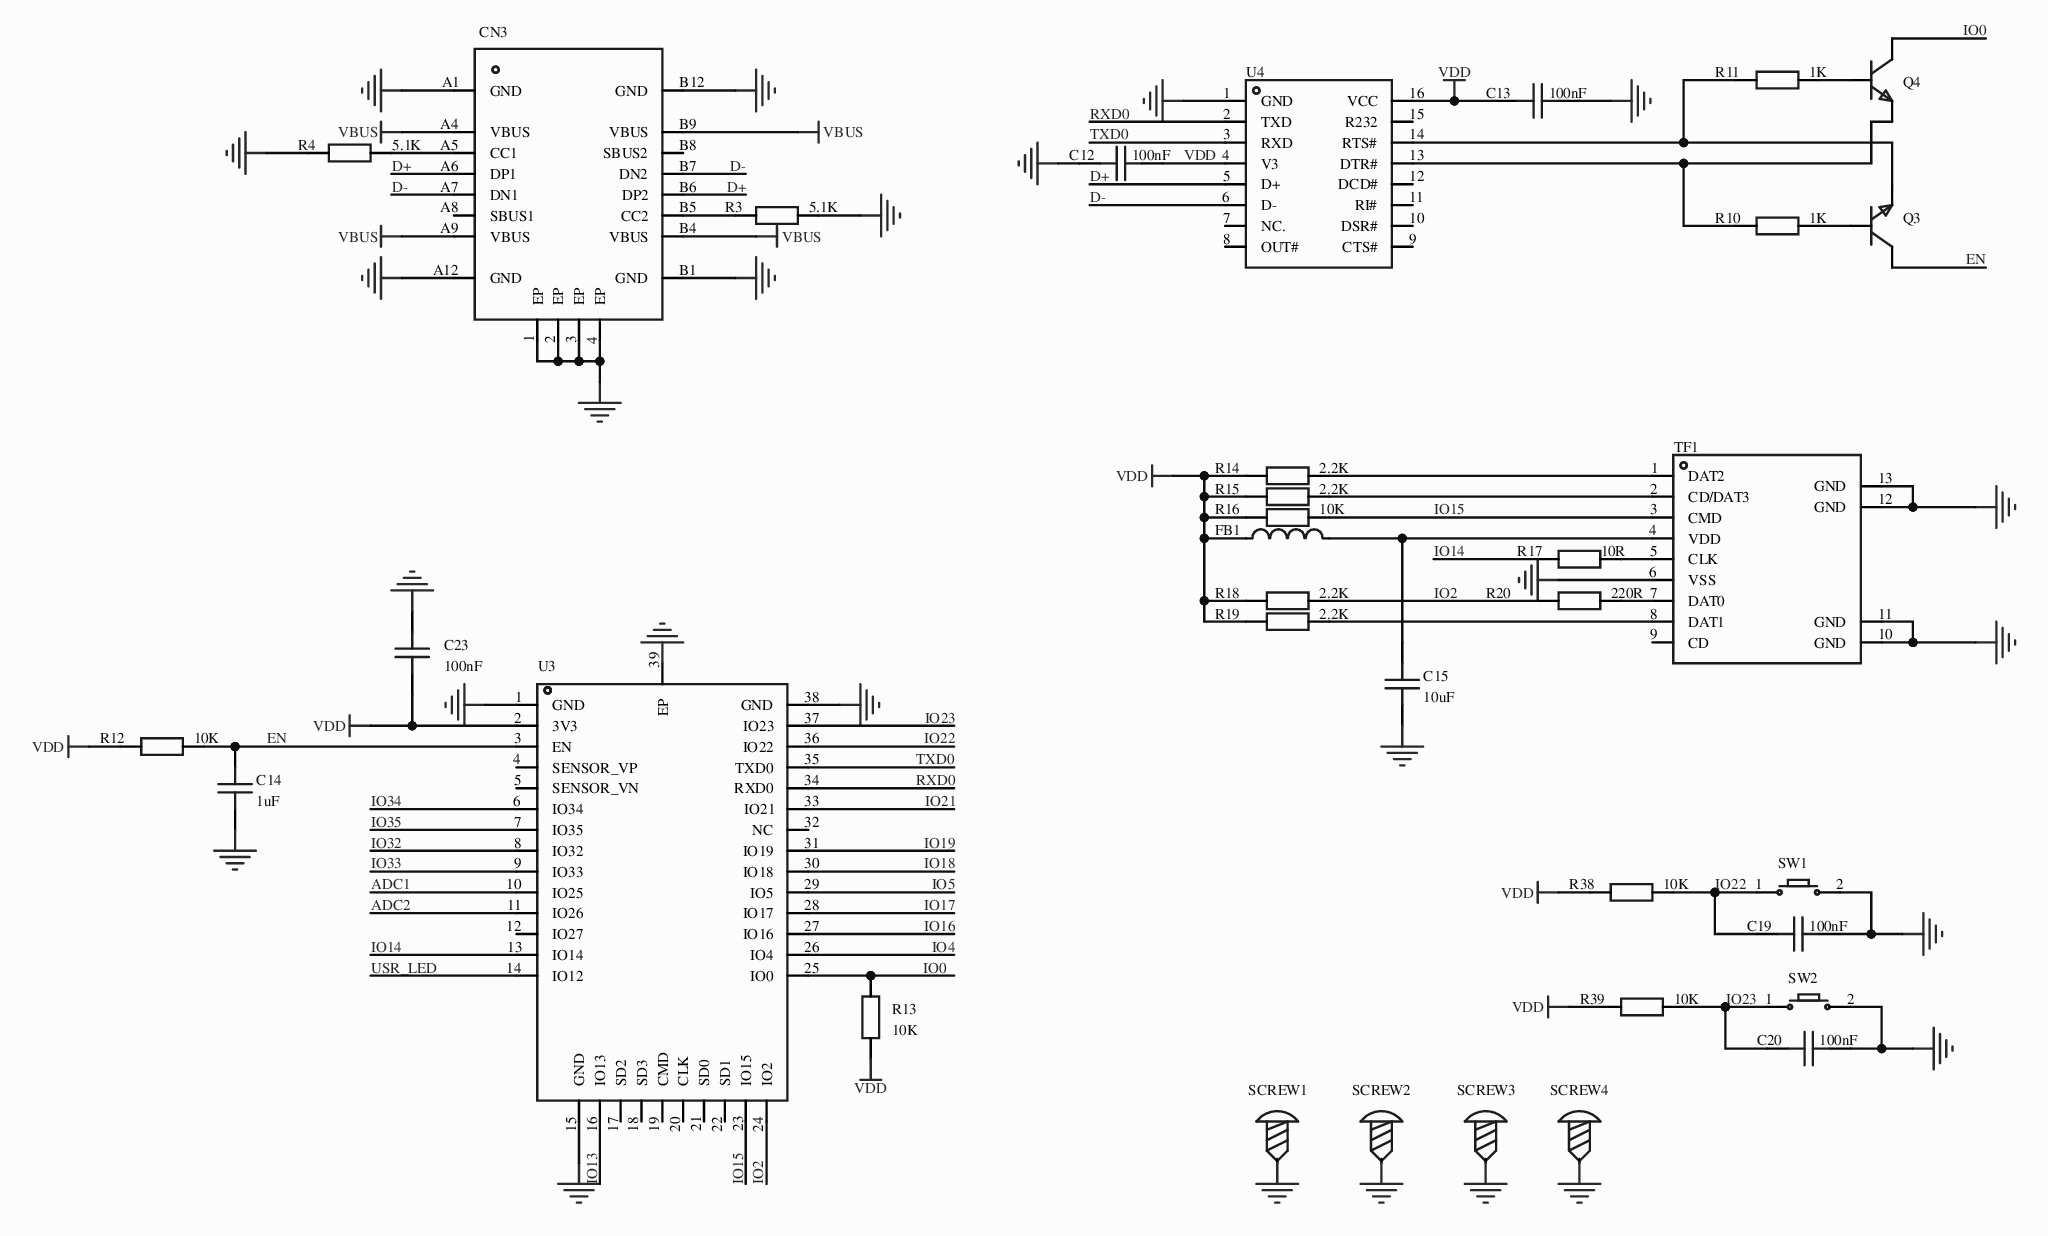
[diagram p0: MISC49869-4.schdoc]
# Altium project MISC49869-2.PrjPcb
3 sheets, 114 parts. Net scope: global (net labels, ports and power ports of the same name join across sheets).
Board file: MISC49869.pcbdoc
Sheets:
  MISC49869-4.schdoc
  MISC49869-3.schdoc
  MISC49869-5.schdoc

## Sheet MISC49869-4.schdoc
size 297 x 209 mm; @Create Time: 11:47:24; @Update Time: 11:51:06; @Board Name: MISC49869; Version: V1.0; @Project Name: MISC49869; @Page Count: 3; @Update Date: 2026-04-07; @Create Date: 2026-04-07; @Schematic Name: MISC49869; @Page No: 1

### Parts
C12  value 100nF  [C0805]  (hidden comment: CAP_0805)
C13  value 100nF  [C0805]  (hidden comment: CAP_0805)
C14  value 1uF  [C0805]  (hidden comment: CAP_0805)
C15  value 10uF  [C0805]  (hidden comment: CAP_0805)
C19  value 100nF  [C0805]  (hidden comment: CAP_0805)
C20  value 100nF  [C0805]  (hidden comment: CAP_0805)
C23  value 100nF  [C0805]  (hidden comment: CAP_0805)
CN3  USB_TYPE-C-16P  [USB_TYPE-C-16P]  (value not drawn)
FB1  L_0805  [L0805]  (value not drawn)
Q3  SS8050_C7420370  [SOT-23-3_L2.9-W1.3-P1.90-LS2.4-BR]  (value not drawn)
Q4  SS8050_C7420370  [SOT-23-3_L2.9-W1.3-P1.90-LS2.4-BR]  (value not drawn)
R3  value 5.1K  [R0805]  (hidden comment: Res_0805)
R4  value 5.1K  [R0805]  (hidden comment: Res_0805)
R10  value 1K  [R0805]  (hidden comment: Res_0805)
R11  value 1K  [R0805]  (hidden comment: Res_0805)
R12  value 10K  [R0805]  (hidden comment: Res_0805)
R13  value 10K  [R0805]  (hidden comment: Res_0805)
R14  value 2.2K  [R0805]  (hidden comment: Res_0805)
R15  value 2.2K  [R0805]  (hidden comment: Res_0805)
R16  value 10K  [R0805]  (hidden comment: Res_0805)
R17  value 10R  [R0805]  (hidden comment: Res_0805)
R18  value 2.2K  [R0805]  (hidden comment: Res_0805)
R19  value 2.2K  [R0805]  (hidden comment: Res_0805)
R20  value 220R  [R0805]  (hidden comment: Res_0805)
R38  value 10K  [R0805]  (hidden comment: Res_0805)
R39  value 10K  [R0805]  (hidden comment: Res_0805)
SCREW1  M2 screw  [M2螺丝]  (value not drawn)
SCREW2  M2 screw  [M2螺丝]  (value not drawn)
SCREW3  M2 screw  [M2螺丝]  (value not drawn)
SCREW4  M2 screw  [M2螺丝]  (value not drawn)
SW1  Key_SMD_3x4x2  [Key_SMD_3x4x2]  (value not drawn)
SW2  Key_SMD_3x4x2  [Key_SMD_3x4x2]  (value not drawn)
TF1  TF-CARD H1.8  [TF-SMD_TF-CARD-H1.8]  (value not drawn)
U3  ESP32-WROOM-32  [WIFIM-SMD_ESP-WROOM-32]  (value not drawn)
U4  CH340C  [SOP-16_L10.0-W3.9-P1.27-LS6.0-BL]  (value not drawn)

### Nets
GND: C12.2 C13.1 C14.2 C15.2 C19.1 C20.1 C23.2 CN3.1(EP) CN3.2(EP) CN3.3(EP) CN3.4(EP) CN3.A1(GND) CN3.A12(GND) CN3.B1(GND) CN3.B12(GND) R3.1 R4.1 SCREW1.1 SCREW2.1 SCREW3.1 SCREW4.1 SW1.2 SW2.2 TF1.6(VSS) TF1.10(GND) TF1.11(GND) TF1.12(GND) TF1.13(GND) U3.1(GND) U3.15(GND) U3.38(GND) U3.39(EP) U4.1(GND)
VBUS: CN3.A4(VBUS) CN3.A9(VBUS) CN3.B4(VBUS) CN3.B9(VBUS)
VDD: C12.1 C13.2 C23.1 FB1.1 R12.2 R13.2 R14.2 R15.2 R16.2 R18.2 R19.2 R38.2 R39.2 U3.2(3V3) U4.4(V3) U4.16(VCC)
ADC1: U3.10(IO25)
ADC2: U3.11(IO26)
D+: CN3.A6(DP1) CN3.B6(DP2) U4.5(D+)
D-: CN3.A7(DN1) CN3.B7(DN2) U4.6(D-)
EN: C14.1 Q3.3(C) R12.1 U3.3(EN)
IO0: Q4.3(C) R13.1 U3.25(IO0)
IO2: R18.1 R20.2 U3.24(IO2)
IO4: U3.26(IO4)
IO5: U3.29(IO5)
IO13: U3.16(IO13)
IO14: R17.2 U3.13(IO14)
IO15: R16.1 TF1.3(CMD) U3.23(IO15)
IO16: U3.27(IO16)
IO17: U3.28(IO17)
IO18: U3.30(IO18)
IO19: U3.31(IO19)
IO21: U3.33(IO21)
IO22: C19.2 R38.1 SW1.1 U3.36(IO22)
IO23: C20.2 R39.1 SW2.1 U3.37(IO23)
IO32: U3.8(IO32)
IO33: U3.9(IO33)
IO34: U3.6(IO34)
IO35: U3.7(IO35)
RXD0: U3.34(RXD0) U4.2(TXD)
TXD0: U3.35(TXD0) U4.3(RXD)
USR_LED: U3.14(IO12)
NetC15_1: C15.1 FB1.2 TF1.4(VDD)
NetCN3_A5: CN3.A5(CC1) R4.2
NetCN3_B5: CN3.B5(CC2) R3.2
NetQ3_1: Q3.1(B) R10.1
NetQ3_2: Q3.2(E) R11.2 U4.14(RTS#)
NetQ4_1: Q4.1(B) R11.1
NetQ4_2: Q4.2(E) R10.2 U4.13(DTR#)
NetR14_1: R14.1 TF1.1(DAT2)
NetR15_1: R15.1 TF1.2(CD/DAT3)
NetR17_1: R17.1 TF1.5(CLK)
NetR19_1: R19.1 TF1.8(DAT1)
NetR20_1: R20.1 TF1.7(DAT0)

Not connected (* = marked no-connect by the designer): CN3 A8(SBUS1)* B8(SBUS2)*; TF1 9(CD)*; U3 4(SENSOR_VP)* 5(SENSOR_VN)* 12(IO27)* 17(SD2)* 18(SD3)* 19(CMD)* 20(CLK)* 21(SD0)* 22(SD1)* 32(NC)*; U4 7(NC.)* 8(OUT#)* 9(CTS#)* 10(DSR#)* 11(RI#)* 12(DCD#)* 15(R232)*

### Library data of the parts
C12-C15 C19 C20 C23 = CAP_0805: ConvertToPcb: yes; SymbolName: CapAcitance; ModelId: 1ba041120af144c991958decab20d241; ModelName: C0805_L2.0-W1.3-H1.3; ModelTransform: 78.74,51.181,0,0,0,0,0,0.0005,0; Device: CAP_0805; AddInBom: yes; FootprintName: C0805
CN3 = USB_TYPE-C-16P: AddInBom: yes; ModelId: 35058e297fd54ee2afd2de30c3ce7155; ModelName: USB-C_SMD-TYPE-C-31-M-12; ModelTransform: 360,318.121,0,180,0,0,0,-41.02,-39.37; Device: USB_TYPE-C-16P; ConvertToPcb: yes; SymbolName: USB_TYPE-C-16P; FootprintName: USB_TYPE-C-16P
FB1 = L_0805: Symbol: SDFL2012S100KTF; Value: 10uH; AddInBom: yes; ModelId: 37a81e68749a4138bd2dfa6897b24b85; ModelName: R0805_L2.0-W1.3-H0.6; ModelTransform: 78.74,51.181,0,0,0,0,0,0.001,0; Device: L_0805; ConvertToPcb: yes; FootprintName: L0805
Q3 Q4 = SS8050_C7420370: AddInBom: yes; ModelId: c62791f0466c4ae2a892c056b845b0ca; ModelName: SOT-23-3P_L2.9-W1.3-H1.0-LS2.4-P0.95; ModelTransform: 98.425,114.173,0,180,0,0,0.0005,-0.0005,0; Symbol: SS8050_C7420370; Device: SS8050_C7420370; ConvertToPcb: yes; FootprintName: SOT-23-3_L2.9-W1.3-P1.90-LS2.4-BR
R3 R4 R10-R20 R38 R39 = Res_0805: ConvertToPcb: yes; SymbolName: Resistor; ModelId: 37a81e68749a4138bd2dfa6897b24b85; ModelName: R0805_L2.0-W1.3-H0.6; ModelTransform: 78.74,51.181,0,0,0,0,0,-0.0005,0; Device: Res_0805; AddInBom: yes; FootprintName: R0805
SCREW1-SCREW4 = M2螺丝: ConvertToPcb: yes; SymbolName: Screw hole; Device: M2 screw; AddInBom: yes; FootprintName: M2 screw
SW1 SW2 = Key_SMD_3x4x2: ConvertToPcb: yes; SymbolName: Tact switch x2; ModelId: 63599cce708d48afbce1b0db003544770819f05c4eef4c71ace90d822a990e87; ModelName: SW-SMD_L4.0-W2.9-H2-LS5.0; ModelTransform: 196.85,114.17,79.13,0,0,0,0,0,0; Device: Key_SMD_3x4x2; AddInBom: yes; FootprintName: Key_SMD_3x4x2
TF1 = TF-CARD H1.8: AddInBom: yes; ModelId: 9b9c093eaf784fafb0b50515d8d92d39; ModelTransform: 631.8885,594.487,0,0,0,0,-0.002,-75.432,-23.622; Symbol: TF-CARD H1.8; Device: TF-CARD H1.8; ConvertToPcb: yes; FootprintName: TF-SMD_TF-CARD-H1.8; ModelName: TF-SMD_TF-CARD-H1.8
U3 = ESP32-WROOM-32: Symbol: ESP-WROOM-32; AddInBom: yes; ModelId: 5a2678a0bdc04ba384e1e7621568aeee; ModelName: WIFIM-SMD_L25.5-W18.0-H3.1; ModelTransform: 709.4474,1004.3287,0,0,0,0,0,145.633,0; Device: ESP32-WROOM-32; ConvertToPcb: yes; FootprintName: WIFIM-SMD_ESP-WROOM-32
U4 = CH340C: AddInBom: yes; ModelId: 3361a6792abf4a8f8fbca4f1924a67ee; ModelName: SOP-16_L9.9-W3.9-H1.5-LS6.0-P1.27; ModelTransform: 240.39054,393.7,0,90,0,0,0,0,0; Symbol: CH340C; Device: CH340C; ConvertToPcb: yes; FootprintName: SOP-16_L10.0-W3.9-P1.27-LS6.0-BL

## Sheet MISC49869-3.schdoc
size 297 x 209 mm; @Create Time: 11:47:24; @Update Time: 09:47:04; @Board Name: MISC49869; Version: V1.0; @Project Name: MISC49869; @Page Count: 3; @Update Date: 2026-04-07; @Create Date: 2026-04-07; @Schematic Name: MISC49869; @Page No: 2
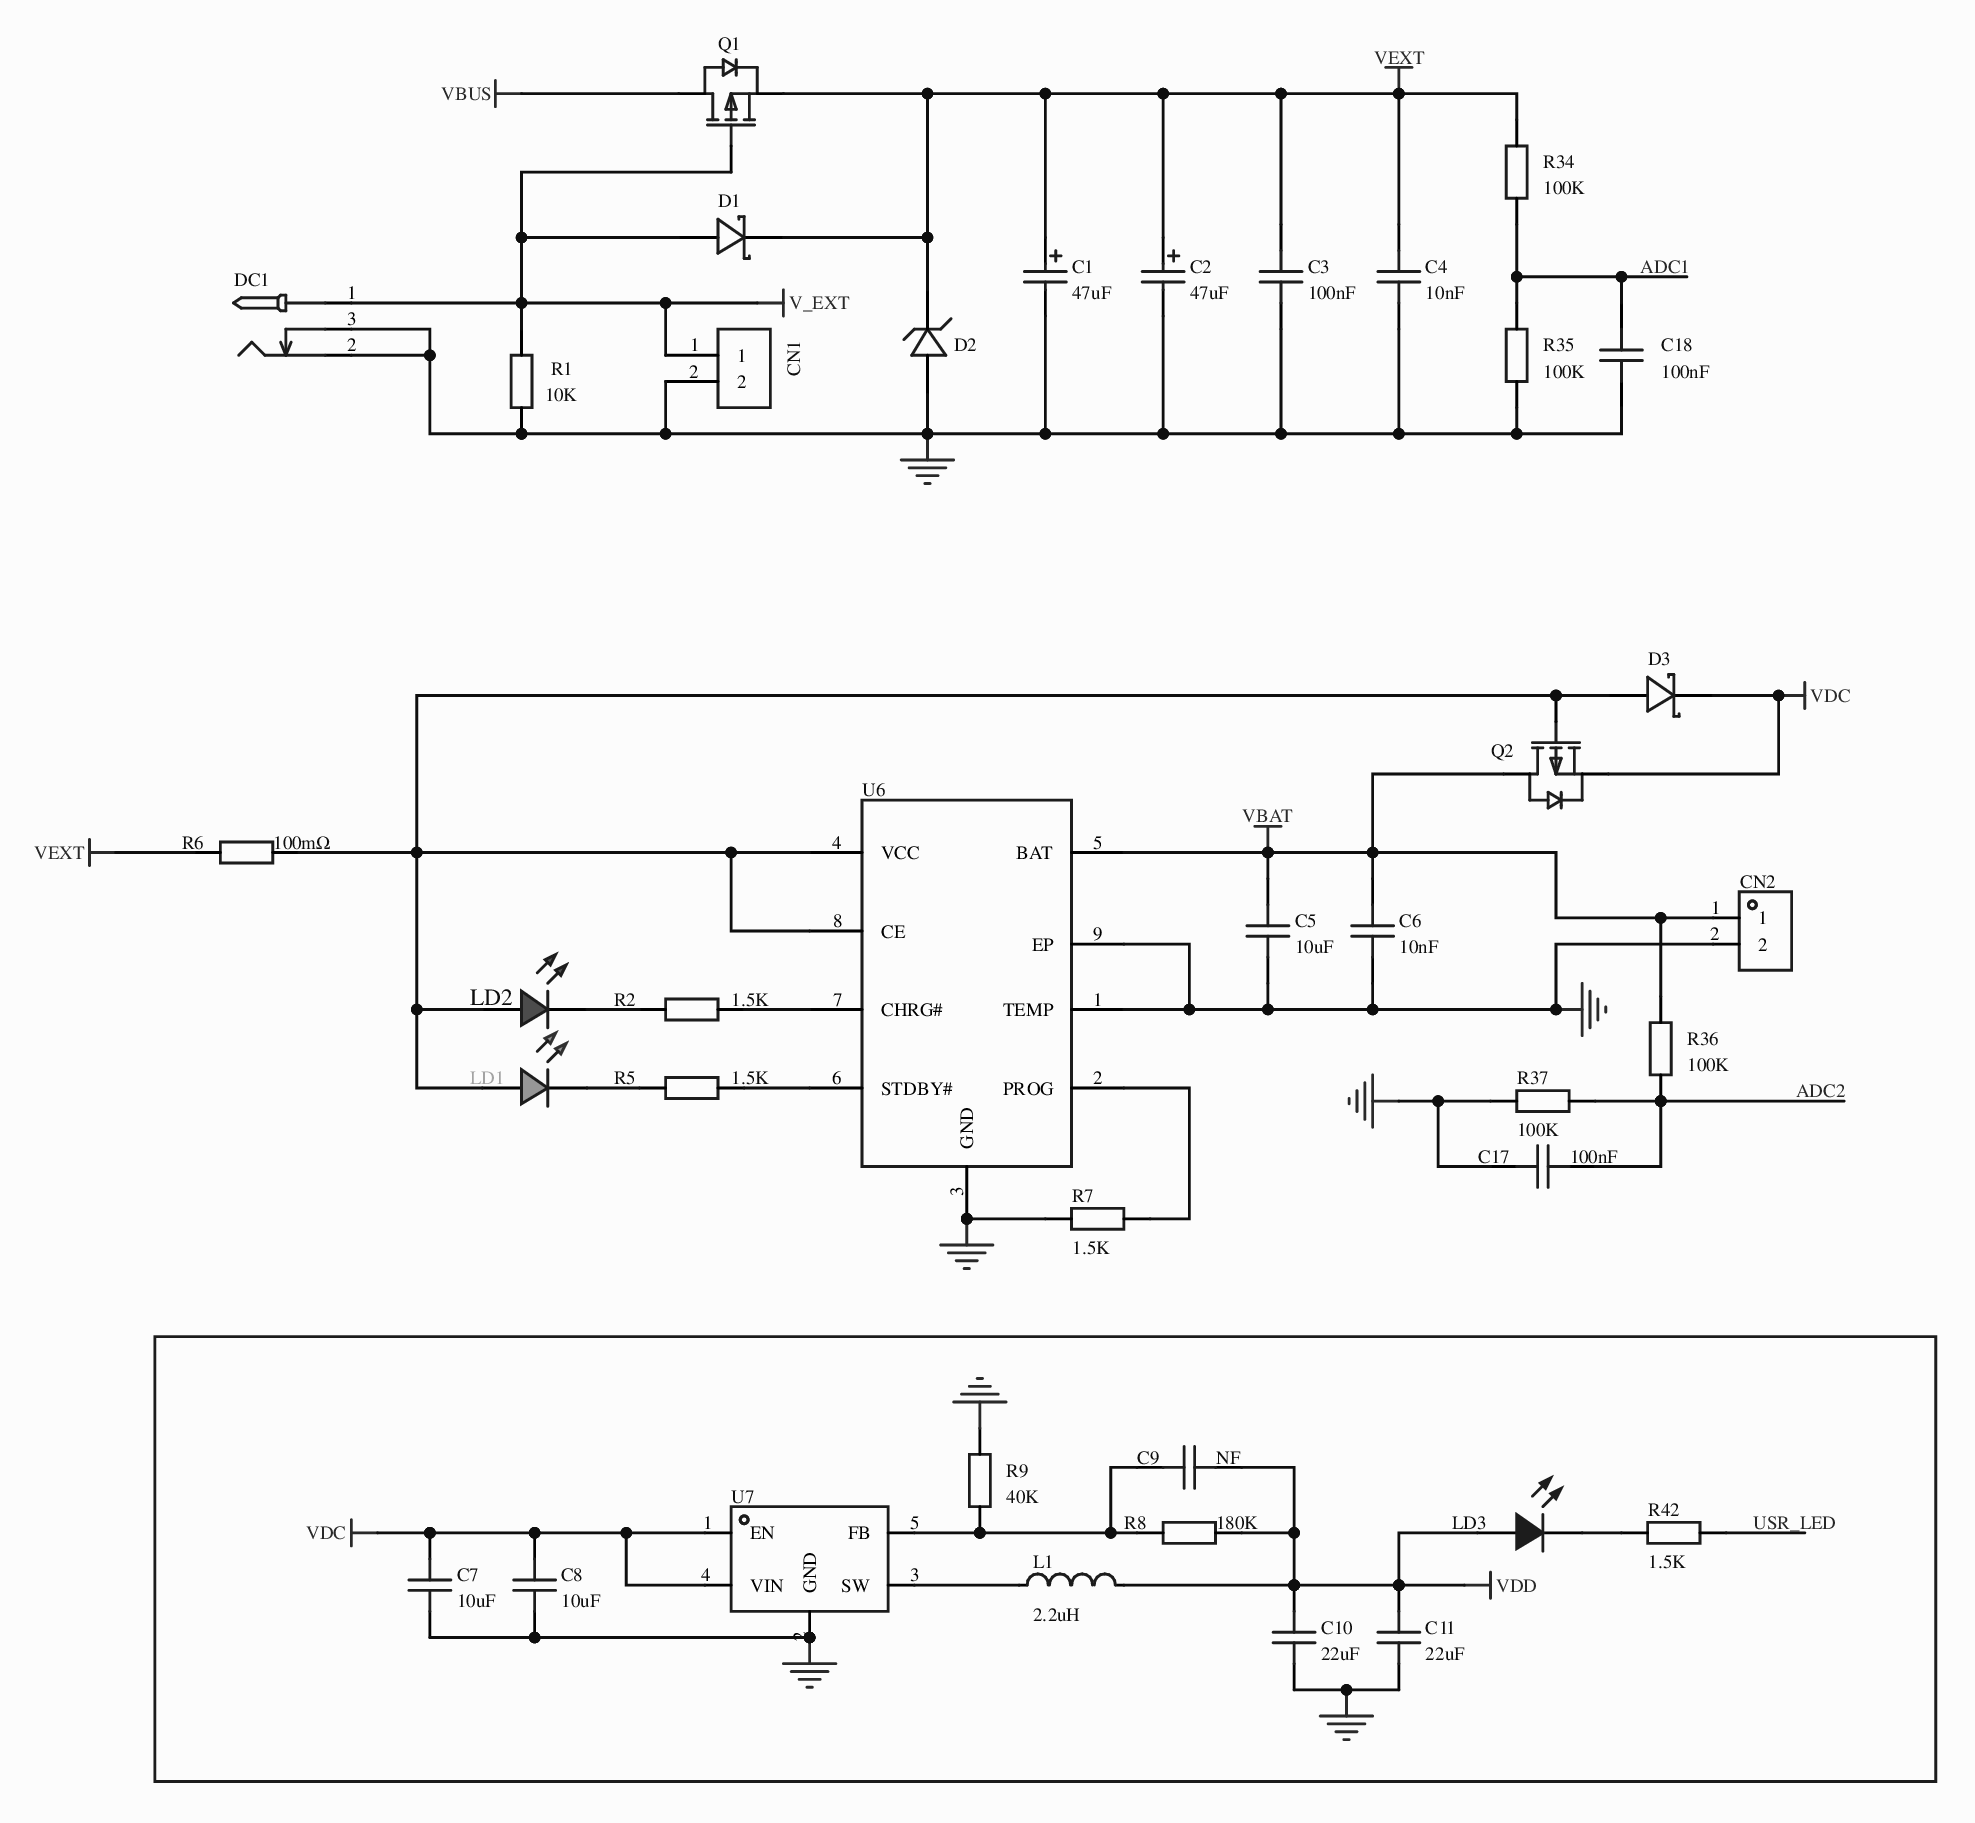
[diagram p1: MISC49869-3.schdoc]

### Parts
C1  value 47uF  [C_Ele_SMD_4x5.5mm]  (hidden comment: C_Ele_SMD_5x5.4mm)
C2  value 47uF  [C_Ele_SMD_4x5.5mm]  (hidden comment: C_Ele_SMD_5x5.4mm)
C3  value 100nF  [C0805]  (hidden comment: CAP_0805)
C4  value 10nF  [C0805]  (hidden comment: CAP_0805)
C5  value 10uF  [C0805]  (hidden comment: CAP_0805)
C6  value 10nF  [C0805]  (hidden comment: CAP_0805)
C7  value 10uF  [C0805]  (hidden comment: CAP_0805)
C8  value 10uF  [C0805]  (hidden comment: CAP_0805)
C9  value NF  [C0805]  (hidden comment: CAP_0805)
C10  value 22uF  [C0805]  (hidden comment: CAP_0805)
C11  value 22uF  [C0805]  (hidden comment: CAP_0805)
C17  value 100nF  [C0805]  (hidden comment: CAP_0805)
C18  value 100nF  [C0805]  (hidden comment: CAP_0805)
CN1  WJ500V-5.08-2P  [CONN-TH_2P-P5.00_WJ500V-5.08-2P]  (value not drawn)
CN2  ZX-XH2.54-2PZZ  [CONN-TH_2P-P2.50_HX25003-2A]  (value not drawn)
D1  SS34_C154551  [SMC_L6.9-W5.9-LS7.9-RD]  (value not drawn)
D2  SMBJ6.0A_C2987966  [SMB_L4.6-W3.6-LS5.3-RD]  (value not drawn)
D3  SS34_C154551  [SMC_L6.9-W5.9-LS7.9-RD]  (value not drawn)
DC1  DC-005_2.5  [DC-005_2.5]  (value not drawn)
L1  value 2.2uH  [IND-SMD_L4.4-W4.2]  (hidden comment: FXL0420-2R2-M)
LD1  LED_0805-G  [LED_0805]  (value not drawn)
LD2  LED_0805-R  [LED_0805]  (value not drawn)
LD3  LED_0805-B  [LED_0805]  (value not drawn)
Q1  AO3401A_C15127  [SOT-23_L2.9-W1.3-P1.90-LS2.4-BR]  (value not drawn)
Q2  AO3401A_C15127  [SOT-23_L2.9-W1.3-P1.90-LS2.4-BR]  (value not drawn)
R1  value 10K  [R0805]  (hidden comment: Res_0805)
R2  value 1.5K  [R0805]  (hidden comment: Res_0805)
R5  value 1.5K  [R0805]  (hidden comment: Res_0805)
R6  value 100mΩ  [R1210]  (hidden comment: 1210W2F100LT5E)
R7  value 1.5K  [R0805]  (hidden comment: Res_0805)
R8  value 180K  [R0805]  (hidden comment: Res_0805)
R9  value 40K  [R0805]  (hidden comment: Res_0805)
R34  value 100K  [R0805]  (hidden comment: Res_0805)
R35  value 100K  [R0805]  (hidden comment: Res_0805)
R36  value 100K  [R0805]  (hidden comment: Res_0805)
R37  value 100K  [R0805]  (hidden comment: Res_0805)
R42  value 1.5K  [R0805]  (hidden comment: Res_0805)
U6  TP4056-42-ESOP8  [ESOP-8_L4.9-W3.9-P1.27-LS6.0-BL-EP]  (value not drawn)
U7  (no value)  [SOT_XDC]

### Nets
GND: C1.2 C2.2 C3.1 C4.1 C5.1 C6.1 C7.1 C8.1 C10.1 C11.1 C17.2 C18.2 CN1.2 CN2.2 D2.2 DC1.2 DC1.3 R1.1 R7.2 R9.1 R35.2 R37.1 U6.1(TEMP) U6.3(GND) U6.9(EP) U7.2(GND)
V_EXT: CN1.1 D1.2(A) DC1.1 Q1.1(G) R1.2
VBAT: C5.2 C6.2 CN2.1 Q2.3(D) R36.2 U6.5(BAT)
VBUS: Q1.3(D)
VDC: C7.2 C8.2 D3.1(C) Q2.2(S) U7.1(EN) U7.4(VIN)
VDD: C9.1 C10.2 C11.2 L1.2 LD3.2(A) R8.2
VEXT: C1.1 C2.1 C3.2 C4.2 D1.1(C) D2.1 Q1.2(S) R6.1 R34.1
ADC1: C18.1 R34.2 R35.1
ADC2: C17.1 R36.1 R37.2
USR_LED: R42.2
NetC9_2: C9.2 R8.1 R9.2 U7.5(FB)
NetD3_2: D3.2(A) LD1.2(A) LD2.2(A) Q2.1(G) R6.2 U6.4(VCC) U6.8(CE)
NetL1_1: L1.1 U7.3(SW)
NetLD1_1: LD1.1(C) R5.2
NetLD2_1: LD2.1(C) R2.2
NetLD3_1: LD3.1(C) R42.1
NetR2_1: R2.1 U6.7(CHRG#)
NetR5_1: R5.1 U6.6(STDBY#)
NetR7_1: R7.1 U6.2(PROG)

### Library data of the parts
C1 C2 = C_Ele_SMD_5x5.4mm: Symbol: CAP; AddInBom: yes; Device: C_Ele_SMD_5x5.4mm; ConvertToPcb: yes; FootprintName: C_Ele_SMD_4x5.5mm
C3-C11 C17 C18 = CAP_0805: as C12 on sheet MISC49869-4; Device: CAP_0805; AddInBom: yes; FootprintName: C0805
CN1 = WJ500V-5.08-2P: Symbol: WJ500V-5.08-2P-14-00A; AddInBom: yes; ModelId: 0f4a503c8d3b4ae19ed61267f5e9a1d7; ModelTransform: 423.621,393.7,0,0,0,0,-11.811,19.685,-137.795; Device: WJ500V-5.08-2P; ConvertToPcb: yes; FootprintName: CONN-TH_2P-P5.00_WJ500V-5.08-2P; ModelName: CONN-TH_2P-P5.00_WJ500V-5.08-2P
CN2 = ZX-XH2.54-2PZZ: AddInBom: yes; ModelId: 17c7be61cc0b4bc5acccb67e71c47088; ModelTransform: 295.275,232.283,0,180,0,0,0,-21.654,-129.921; Symbol: ZX-XH2.54-2PZZ; Device: ZX-XH2.54-2PZZ; ConvertToPcb: yes; FootprintName: CONN-TH_2P-P2.50_HX25003-2A; ModelName: CONN-TH_2P-P2.50_HX25003-2A
D1 D3 = SS34_C154551: AddInBom: yes; ModelId: 4f14ab132b494223bc17c7f39616ac35; ModelTransform: 314.96,236.22,0,0,0,0,0,0,0; Symbol: SS34_C154551; Device: SS34_C154551; ConvertToPcb: yes; FootprintName: SMC_L6.9-W5.9-LS7.9-RD; ModelName: SMC_L6.9-W5.9-LS7.9-RD
D2 = SMBJ6.0A_C2987966: AddInBom: yes; ModelId: 5e8926c661484ff2a35b83e5ae62aeb9; ModelTransform: 212.598,141.732,0,0,0,0,0,0,0; Symbol: SMBJ6.0A_C2987966; Device: SMBJ6.0A_C2987966; ConvertToPcb: yes; FootprintName: SMB_L4.6-W3.6-LS5.3-RD; ModelName: SMB_L4.6-W3.6-LS5.3-RD
DC1 = DC-005_2.5: ConvertToPcb: yes; ModelId: f168fe383f964e0ea2af0127ff6ac7b40819f05c4eef4c71ace90d822a990e87; ModelName: DC-IN-TH_DC005; ModelTransform: 366.14,553.15,590.55,90,0,0,137.8,-11.81,-157.48; Device: DC-005_2.5; AddInBom: yes; SymbolName: DC-005_2.5; FootprintName: DC-005_2.5
L1 = FXL0420-2R2-M: AddInBom: yes; ModelId: e9b3d3f4fa134185b54d517730715f16; ModelName: IND-SMD_L4.2-W4.4-H2.0; ModelTransform: 173.228,165.354,0,0,0,0,0,0,0; Tolerance: ±20%; Symbol: FXL0420-2R2-M; Device: FXL0420-2R2-M; ConvertToPcb: yes; FootprintName: IND-SMD_L4.4-W4.2
LD1 = LED_0805-G: Symbol: LED_G; Convert to PCB: yes; 3D Model: 381ae4d721d6485eaad9d0ca067812b5; 3D Model Transform: 63.9,39.8,31.9,0,0,0,0,0,0; ModelName: LED-0805_G; Device: LED_0805-G; Add into BOM: yes; FootprintName: LED_0805
LD2 = LED_0805-R: Symbol: LED_R; Convert to PCB: yes; 3D Model: 33fb9fca58e84f37a403ebeef4c28b77; 3D Model Transform: 78.7,49.1,39.3,0,0,0,0,0,0; ModelName: LED-0805_R; Device: LED_0805-R; Add into BOM: yes; FootprintName: LED_0805
LD3 = LED_0805-B: Symbol: LED_B; Convert to PCB: yes; 3D Model: 15b3689d29af4f66b19acfbf3642d2c8; 3D Model Transform: 79,49.2,39.4,0,0,0,0,0,0; ModelName: LED-0805_B; Device: LED_0805-B; Add into BOM: yes; FootprintName: LED_0805
Q1 Q2 = AO3401A_C15127: AddInBom: yes; ModelId: c62791f0466c4ae2a892c056b845b0ca; ModelName: SOT-23-3P_L2.9-W1.3-H1.0-LS2.4-P0.95; ModelTransform: 98.64468,114.173,0,180,0,0,0,0,0; Symbol: AO3401A; Device: AO3401A_C15127; ConvertToPcb: yes; FootprintName: SOT-23_L2.9-W1.3-P1.90-LS2.4-BR
R1 R2 R5 R7-R9 R34-R37 R42 = Res_0805: as R3 on sheet MISC49869-4; Device: Res_0805; AddInBom: yes; FootprintName: R0805
R6 = 1210W2F100LT5E: AddInBom: yes; ModelId: beebf7deb00343bea1f9ba031f1dd141; ModelName: R1210_L3.2-W2.6-H0.6; ModelTransform: 125.984,102.362,0,0,0,0,0,0,0; Tolerance: ±1%; Symbol: 1210W2F100LT5E; Device: 1210W2F100LT5E; ConvertToPcb: yes; FootprintName: R1210
U6 = TP4056-42-ESOP8: Symbol: TP4056; AddInBom: yes; ModelId: d3e00daa36c445139c055a3b9efb85d2; ModelName: ESOP-8_L4.9-W3.9-H1.6-LS6.0-P1.27; ModelTransform: 240.157,192.913,0,90,0,0,0,0,0; Device: TP4056-42-ESOP8; ConvertToPcb: yes; FootprintName: ESOP-8_L4.9-W3.9-P1.27-LS6.0-BL-EP
U7 = XDC: AddInBom: yes; Device: XDC; SymbolName: XDC; ConvertToPcb: yes

## Sheet MISC49869-5.schdoc
size 297 x 209 mm; @Create Time: 11:47:24; @Update Time: 15:50:24; @Board Name: MISC49869; Version: V1.0; @Project Name: MISC49869; @Page Count: 3; @Update Date: 2026-04-07; @Create Date: 2026-04-07; @Schematic Name: MISC49869; @Page No: 3
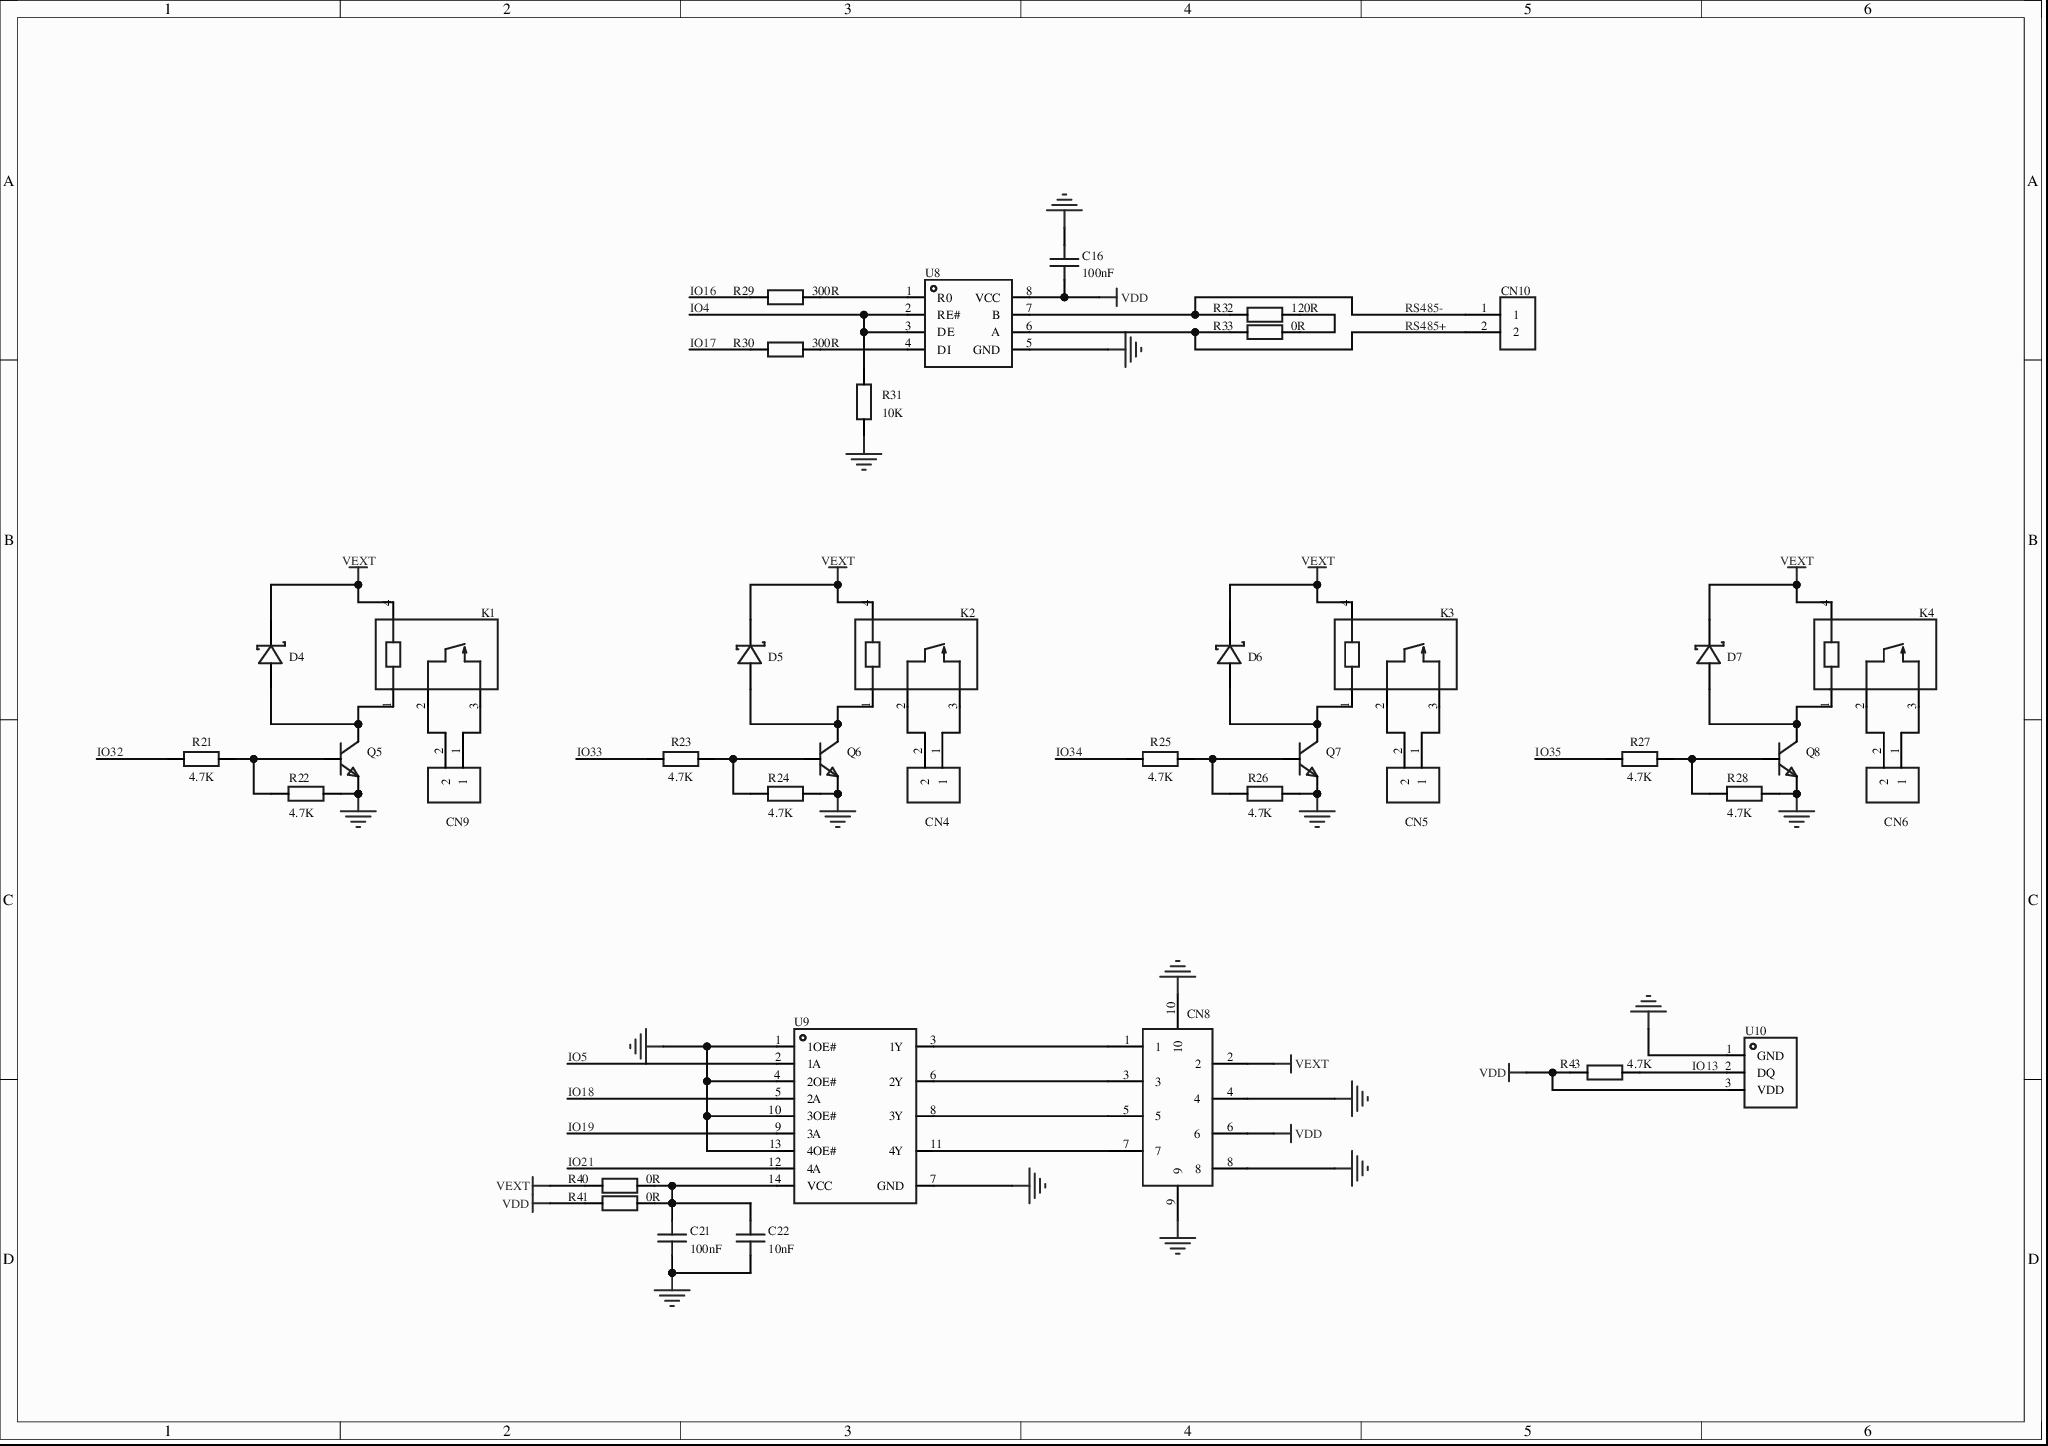
[diagram p2: MISC49869-5.schdoc]

### Parts
C16  value 100nF  [C0805]  (hidden comment: CAP_0805)
C21  value 100nF  [C0805]  (hidden comment: CAP_0805)
C22  value 10nF  [C0805]  (hidden comment: CAP_0805)
CN4  WJ500V-5.08-2P  [CONN-TH_2P-P5.00_WJ500V-5.08-2P]  (value not drawn)
CN5  WJ500V-5.08-2P  [CONN-TH_2P-P5.00_WJ500V-5.08-2P]  (value not drawn)
CN6  WJ500V-5.08-2P  [CONN-TH_2P-P5.00_WJ500V-5.08-2P]  (value not drawn)
CN8  8P-SMD with latch  [FPC-SMD_8P-P0.50_AFC11-S08ICC-00]  (value not drawn)
CN9  WJ500V-5.08-2P  [CONN-TH_2P-P5.00_WJ500V-5.08-2P]  (value not drawn)
CN10  WJ500V-5.08-2P  [CONN-TH_2P-P5.00_WJ500V-5.08-2P]  (value not drawn)
D4  SS34_C154551  [SMC_L6.9-W5.9-LS7.9-RD]  (value not drawn)
D5  SS34_C154551  [SMC_L6.9-W5.9-LS7.9-RD]  (value not drawn)
D6  SS34_C154551  [SMC_L6.9-W5.9-LS7.9-RD]  (value not drawn)
D7  SS34_C154551  [SMC_L6.9-W5.9-LS7.9-RD]  (value not drawn)
K1  G5NB-1A-E-12VDC  [RELAY-TH_G5NB-1A-E-DCXX]  (value not drawn)
K2  G5NB-1A-E-12VDC  [RELAY-TH_G5NB-1A-E-DCXX]  (value not drawn)
K3  G5NB-1A-E-12VDC  [RELAY-TH_G5NB-1A-E-DCXX]  (value not drawn)
K4  G5NB-1A-E-12VDC  [RELAY-TH_G5NB-1A-E-DCXX]  (value not drawn)
Q5  SS8050_C7420370  [SOT-23-3_L2.9-W1.3-P1.90-LS2.4-BR]  (value not drawn)
Q6  SS8050_C7420370  [SOT-23-3_L2.9-W1.3-P1.90-LS2.4-BR]  (value not drawn)
Q7  SS8050_C7420370  [SOT-23-3_L2.9-W1.3-P1.90-LS2.4-BR]  (value not drawn)
Q8  SS8050_C7420370  [SOT-23-3_L2.9-W1.3-P1.90-LS2.4-BR]  (value not drawn)
R21  value 4.7K  [R0805]  (hidden comment: Res_0805)
R22  value 4.7K  [R0805]  (hidden comment: Res_0805)
R23  value 4.7K  [R0805]  (hidden comment: Res_0805)
R24  value 4.7K  [R0805]  (hidden comment: Res_0805)
R25  value 4.7K  [R0805]  (hidden comment: Res_0805)
R26  value 4.7K  [R0805]  (hidden comment: Res_0805)
R27  value 4.7K  [R0805]  (hidden comment: Res_0805)
R28  value 4.7K  [R0805]  (hidden comment: Res_0805)
R29  value 300R  [R0805]  (hidden comment: Res_0805)
R30  value 300R  [R0805]  (hidden comment: Res_0805)
R31  value 10K  [R0805]  (hidden comment: Res_0805)
R32  value 120R  [R0805]  (hidden comment: Res_0805)
R33  value 0R  [R0805]  (hidden comment: Res_0805)
R40  value 0R  [R0805]  (hidden comment: Res_0805)
R41  value 0R  [R0805]  (hidden comment: Res_0805)
R43  value 4.7K  [R0805]  (hidden comment: Res_0805)
U8  MAX485EIM/TR  [SOP-8_L4.9-W3.9-P1.27-LS6.0-BL]  (value not drawn)
U9  74HC125D/S400118  [SOIC-14_L8.6-W3.8-P1.27-LS6.0-BL]  (value not drawn)
U10  (no value)  [TO-92-3_L4.9-W3.7-P1.27-L]

### Nets
GND: C16.2 C21.1 C22.1 CN8.4 CN8.8 CN8.9 CN8.10 Q5.2(E) Q6.2(E) Q7.2(E) Q8.2(E) R22.1 R24.1 R26.1 R28.1 R31.2 U8.5(GND) U9.1(1OE#) U9.4(2OE#) U9.7(GND) U9.10(3OE#) U9.13(4OE#) U10.1(GND)
VDD: C16.1 CN8.6 R41.2 R43.2 U8.8(VCC) U10.3(VDD)
VEXT: CN8.2 D4.1(C) D5.1(C) D6.1(C) D7.1(C) K1.4 K2.4 K3.4 K4.4 R40.2
IO4: R31.1 U8.2(RE#) U8.3(DE)
IO5: U9.2(1A)
IO13: R43.1 U10.2(DQ)
IO16: R29.2
IO17: R30.2
IO18: U9.5(2A)
IO19: U9.9(3A)
IO21: U9.12(4A)
IO32: R21.2
IO33: R23.2
IO34: R25.2
IO35: R27.2
RS485+: CN10.2 R33.1 U8.6(A)
RS485-: CN10.1 R32.1 U8.7(B)
NetC21_2: C21.2 C22.2 R40.1 R41.1 U9.14(VCC)
NetCN4_1: CN4.1 K2.3
NetCN4_2: CN4.2 K2.2
NetCN5_1: CN5.1 K3.3
NetCN5_2: CN5.2 K3.2
NetCN6_1: CN6.1 K4.3
NetCN6_2: CN6.2 K4.2
NetCN8_1: CN8.1 U9.3(1Y)
NetCN8_3: CN8.3 U9.6(2Y)
NetCN8_5: CN8.5 U9.8(3Y)
NetCN8_7: CN8.7 U9.11(4Y)
NetCN9_1: CN9.1 K1.3
NetCN9_2: CN9.2 K1.2
NetD4_2: D4.2(A) K1.1 Q5.3(C)
NetD5_2: D5.2(A) K2.1 Q6.3(C)
NetD6_2: D6.2(A) K3.1 Q7.3(C)
NetD7_2: D7.2(A) K4.1 Q8.3(C)
NetQ5_1: Q5.1(B) R21.1 R22.2
NetQ6_1: Q6.1(B) R23.1 R24.2
NetQ7_1: Q7.1(B) R25.1 R26.2
NetQ8_1: Q8.1(B) R27.1 R28.2
NetR29_1: R29.1 U8.1(R0)
NetR30_1: R30.1 U8.4(DI)
NetR32_2: R32.2 R33.2

### Library data of the parts
C16 C21 C22 = CAP_0805: as C12 on sheet MISC49869-4; Device: CAP_0805; AddInBom: yes; FootprintName: C0805
CN4-CN6 CN9 CN10 = WJ500V-5.08-2P: as CN1 on sheet MISC49869-3; Device: WJ500V-5.08-2P; ConvertToPcb: yes; FootprintName: CONN-TH_2P-P5.00_WJ500V-5.08-2P; ModelName: CONN-TH_2P-P5.00_WJ500V-5.08-2P
CN8 = 8P-立贴带锁: AddInBom: yes; ModelId: c1555c9be5f54c84928632d14a08c4dc; ModelTransform: 377.952,118.11,0,0,0,0,0,0,0; Symbol: 8P-SMD with latch; Device: 8P-SMD with latch; ConvertToPcb: yes; FootprintName: FPC-SMD_8P-P0.50_AFC11-S08ICC-00; ModelName: FPC-SMD_8P-P0.50_AFC11-S08ICC-00
D4-D7 = SS34_C154551: as D1 on sheet MISC49869-3; Symbol: SS34_C154551; Device: SS34_C154551; ConvertToPcb: yes; FootprintName: SMC_L6.9-W5.9-LS7.9-RD; ModelName: SMC_L6.9-W5.9-LS7.9-RD
K1-K4 = G5NB-1A-E-12VDC: AddInBom: yes; ModelId: 6120fb8104464971ad0bbab563986a92; ModelName: RELAY-TH_L20.5-W7.0-H15.0; ModelTransform: 807.085,275.984,0,0,0,0,-0.002,-0.001,-118.11; Symbol: G5NB-1A-E-12VDC; Device: G5NB-1A-E-12VDC; ConvertToPcb: yes; FootprintName: RELAY-TH_G5NB-1A-E-DCXX
Q5-Q8 = SS8050_C7420370: as Q3 on sheet MISC49869-4; Symbol: SS8050_C7420370; Device: SS8050_C7420370; ConvertToPcb: yes; FootprintName: SOT-23-3_L2.9-W1.3-P1.90-LS2.4-BR
R21-R33 R40 R41 R43 = Res_0805: as R3 on sheet MISC49869-4; Device: Res_0805; AddInBom: yes; FootprintName: R0805
U8 = MAX485EIM/TR: AddInBom: yes; ModelId: 75c24a7891ee4dd6bdac16a7163ff87e; ModelName: SOP-8_L4.9-W3.9-P1.27-LS6.0-BL-1; ModelTransform: 192.913,236.22,0,0,0,0,0,0,0; Symbol: MAX485EIM/TR; Device: MAX485EIM/TR; ConvertToPcb: yes; FootprintName: SOP-8_L4.9-W3.9-P1.27-LS6.0-BL
U9 = 74HC125D/S400118: AddInBom: yes; ModelId: 8472f5b0db2b4280be1c9908280b498e; ModelTransform: 340.5505,236.22,0,0,0,0,0,0,0; Symbol: 74HC125D/S400118; Device: 74HC125D/S400118; ConvertToPcb: yes; FootprintName: SOIC-14_L8.6-W3.8-P1.27-LS6.0-BL; ModelName: SOIC-14_L8.6-W3.8-P1.27-LS6.0-BL
U10 = GX18B20: AddInBom: yes; ModelId: aafe8e06f2154e7c93506efd0d6632dd; ModelTransform: 180.7872,141.4455,0,0,0,0,0,22.677,-196.85; Device: GX18B20; Symbol: GX18B20; ConvertToPcb: yes; FootprintName: TO-92-3_L4.9-W3.7-P1.27-L; ModelName: TO-92-3_L4.9-W3.7-P1.27-L; Sensor Type: -; Output Type: -; Sensing Temperature-Local: -; Sensing Temperature-remote: -; Resolution: -; Features: -; Voltage-Supply: -; Accuracy-Highest(lowest): -; Operating Temperature: -

## Nets that join several sheets
GND: MISC49869-4 (33 pins), MISC49869-3 (26 pins), MISC49869-5 (23 pins)
VBUS: MISC49869-4 (CN3.A4 CN3.A9 CN3.B4 CN3.B9), MISC49869-3 (Q1.3)
VDD: MISC49869-4 (16 pins), MISC49869-3 (6 pins), MISC49869-5 (6 pins)
VEXT: MISC49869-3 (9 pins), MISC49869-5 (10 pins)
ADC1: MISC49869-4 (U3.10), MISC49869-3 (C18.1 R34.2 R35.1)
ADC2: MISC49869-4 (U3.11), MISC49869-3 (C17.1 R36.1 R37.2)
IO4: MISC49869-4 (U3.26), MISC49869-5 (R31.1 U8.2 U8.3)
IO5: MISC49869-4 (U3.29), MISC49869-5 (U9.2)
IO13: MISC49869-4 (U3.16), MISC49869-5 (R43.1 U10.2)
IO16: MISC49869-4 (U3.27), MISC49869-5 (R29.2)
IO17: MISC49869-4 (U3.28), MISC49869-5 (R30.2)
IO18: MISC49869-4 (U3.30), MISC49869-5 (U9.5)
IO19: MISC49869-4 (U3.31), MISC49869-5 (U9.9)
IO21: MISC49869-4 (U3.33), MISC49869-5 (U9.12)
IO32: MISC49869-4 (U3.8), MISC49869-5 (R21.2)
IO33: MISC49869-4 (U3.9), MISC49869-5 (R23.2)
IO34: MISC49869-4 (U3.6), MISC49869-5 (R25.2)
IO35: MISC49869-4 (U3.7), MISC49869-5 (R27.2)
USR_LED: MISC49869-4 (U3.14), MISC49869-3 (R42.2)